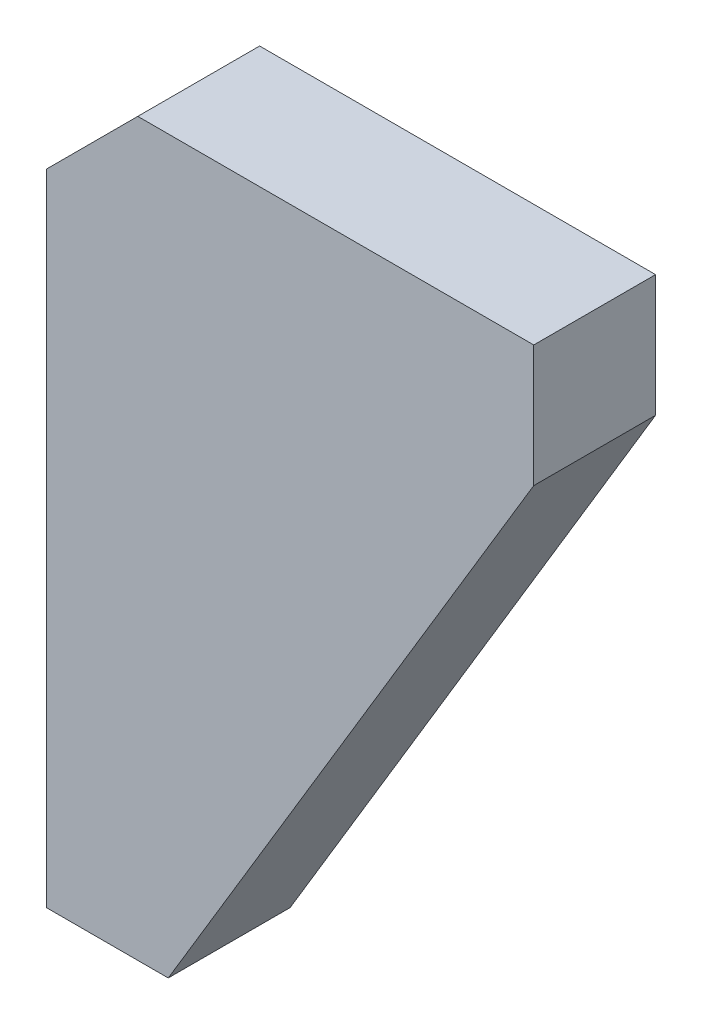
SolidWorks part; units mm, degrees
ref_plane "Front Plane" through (0, 0, 0) normal (0, 0, 1) x (1, 0, 0)
ref_plane "Top Plane" through (0, 0, 0) normal (0, 1, 0) x (1, 0, 0)
ref_plane "Right Plane" through (0, 0, 0) normal (1, 0, 0) x (0, 0, -1)
sketch "Sketch1" plane through (0, 0, 0) normal (0, 0, 1) x (1, 0, 0)
  line L0 (0, 0) -> (0, 105)
  line L1 (15, 120) -> (80, 120)
  line L2 (80, 120) -> (80, 100)
  line L3 (80, 100) -> (20, 0)
  line L4 (20, 0) -> (0, 0)
  line L5 (0, 105) -> (15, 120)
  point P1 (0, 120)
  dimension "D1" = 120
  dimension "D2" = 20
  dimension "D3" = 20
  dimension "D4" = 80
extrude "Boss-Extrude1" add sketch "Sketch1" along normal blind 20
